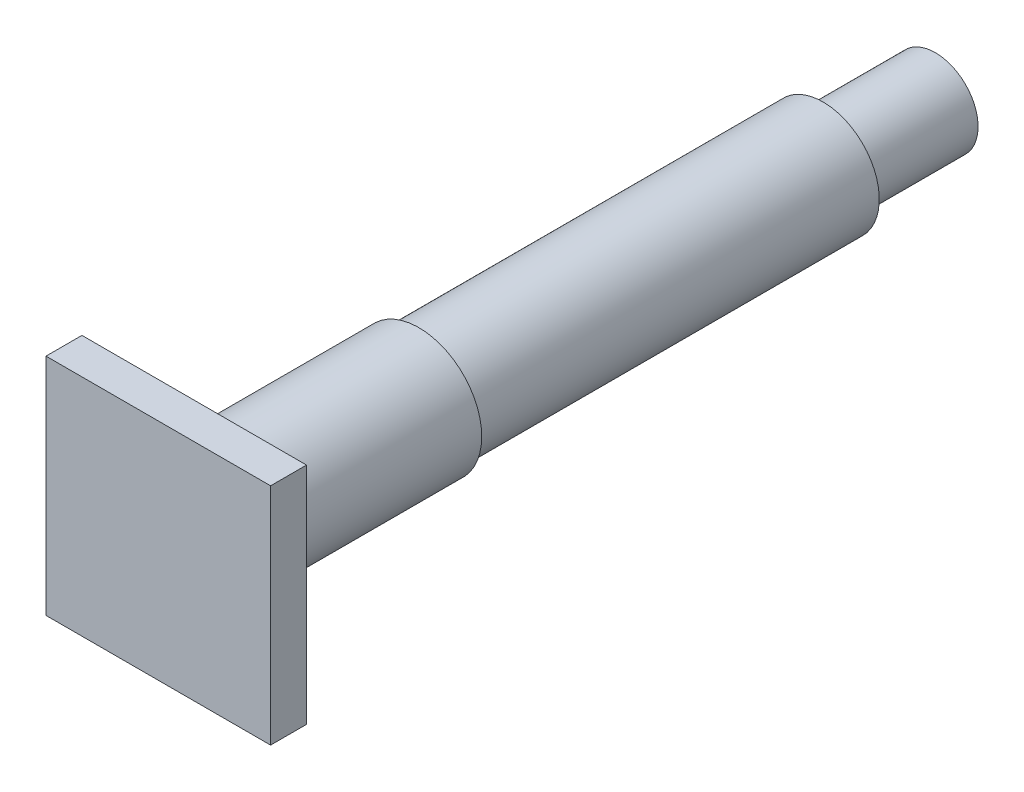
from build123d import *

# Parameters (mm, degrees)
SKETCH_1_R      = 12.5
EXTRUDE_1_DEPTH = 90
SKETCH_2_R      = 14
EXTRUDE_2_DEPTH = 50
SKETCH_3_W      = 50
SKETCH_3_H      = 50
EXTRUDE_3_DEPTH = 8
SKETCH_4_R      = 9.5
EXTRUDE_4_DEPTH = 25


with BuildPart() as part:
    # 草图1 → 凸台-拉伸1 (new body)
    with BuildSketch(Plane.XY):
        with Locations(Location((0, 0, 0), (0, 0, 180))):
            Circle(SKETCH_1_R)
    extrude(amount=EXTRUDE_1_DEPTH)

    # 草图2 → 凸台-拉伸2 (add)
    with BuildSketch(Plane.XY.offset(90)):
        Circle(SKETCH_2_R)
    extrude(amount=EXTRUDE_2_DEPTH)

    # 草图3 → 凸台-拉伸3 (add)
    with BuildSketch(Plane.XY.offset(140)):
        Rectangle(SKETCH_3_W, SKETCH_3_H)
    extrude(amount=EXTRUDE_3_DEPTH)

    # 草图4 → 凸台-拉伸4 (add)
    with BuildSketch(Plane(origin=(0, 0, 0), x_dir=(-1, 0, 0), z_dir=(0, 0, -1))):
        Circle(SKETCH_4_R)
    extrude(amount=EXTRUDE_4_DEPTH)


solid = part.part
